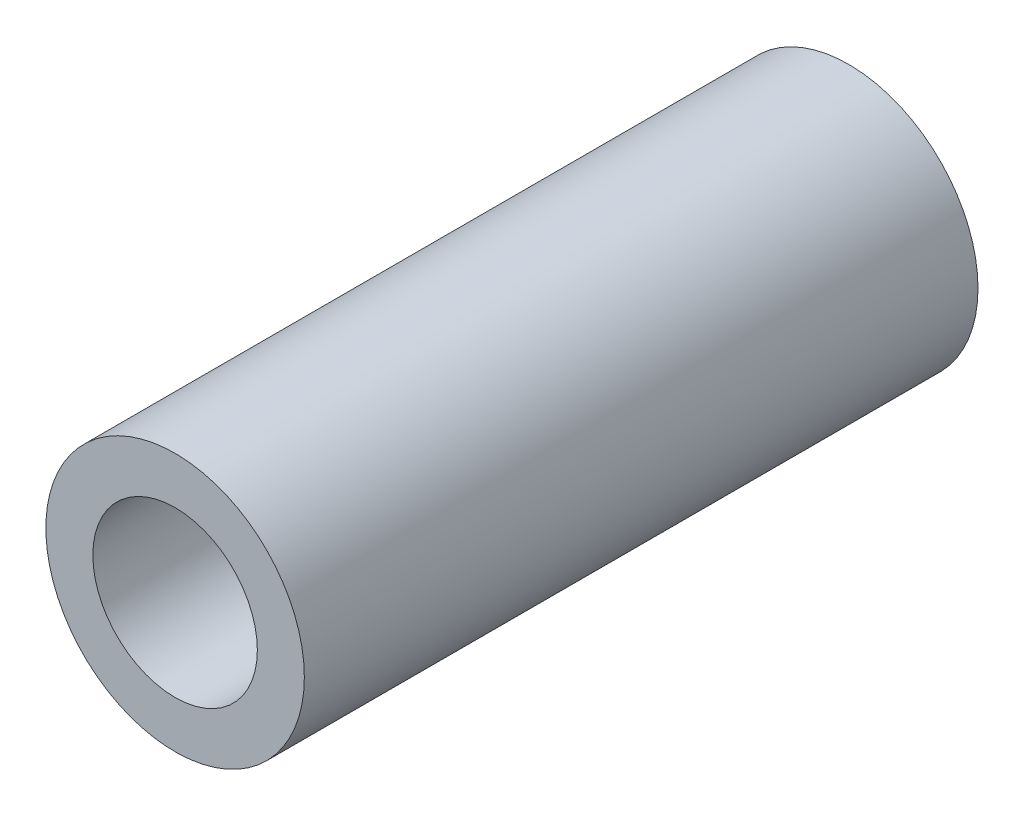
SolidWorks part; units mm, degrees
material "-"
ref_plane "Front Plane" through (0, 0, 0) normal (0, 0, 1) x (1, 0, 0)
ref_plane "Top Plane" through (0, 0, 0) normal (0, 1, 0) x (1, 0, 0)
ref_plane "Right Plane" through (0, 0, 0) normal (1, 0, 0) x (0, 0, -1)
sketch "Sketch1" plane through (0, 0, 0) normal (0, 0, 1) x (1, 0, 0)
  circle A1 centre (0, 0) radius 8.25
  dimension "D2" = 16.5
extrude "Boss-Extrude1" add sketch "Sketch1" along normal blind 43
sketch "Sketch2" plane through (0, 0, 43) normal (0, 0, 1) x (1, 0, 0)
  circle A0 centre (0, 0) radius 5.25
  dimension "D1" = 10.5
extrude "Cut-Extrude1" cut sketch "Sketch2" against normal blind 100
